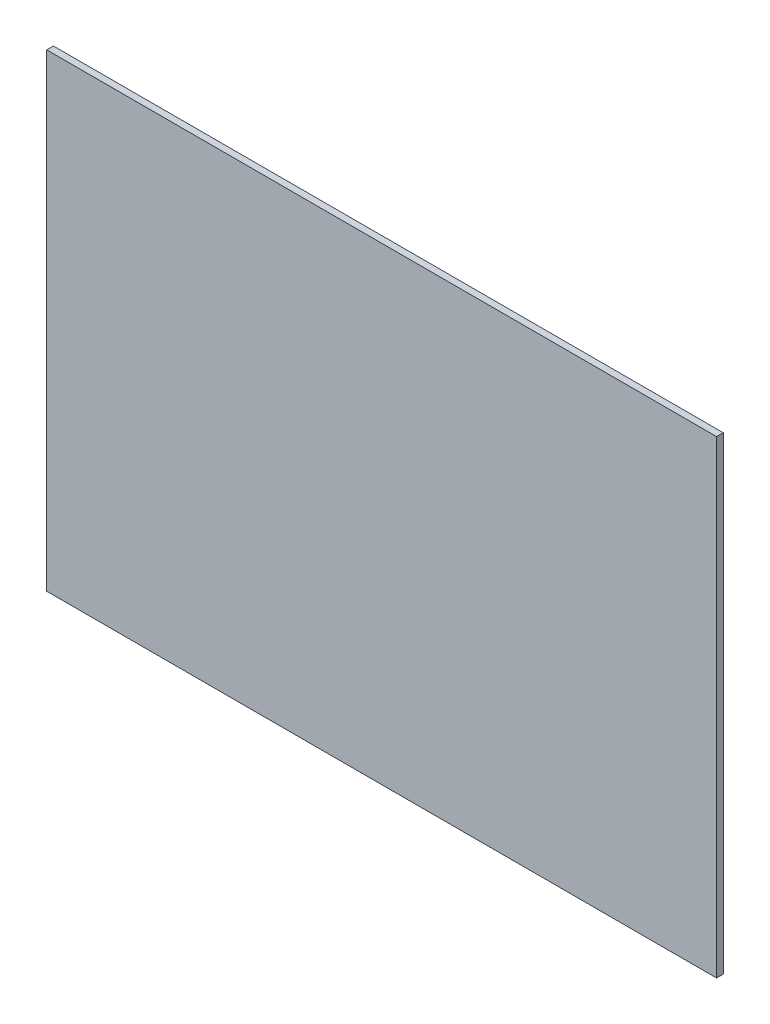
from build123d import *

# Parameters (mm, degrees)
SKETCH1_W           = 1000
SKETCH1_H           = 700
BOSS_EXTRUDE1_DEPTH = 10


with BuildPart() as part:
    # Sketch1 → Boss-Extrude1 (new body)
    with BuildSketch(Plane.XY):
        Rectangle(SKETCH1_W, SKETCH1_H)
    extrude(amount=BOSS_EXTRUDE1_DEPTH)


solid = part.part
